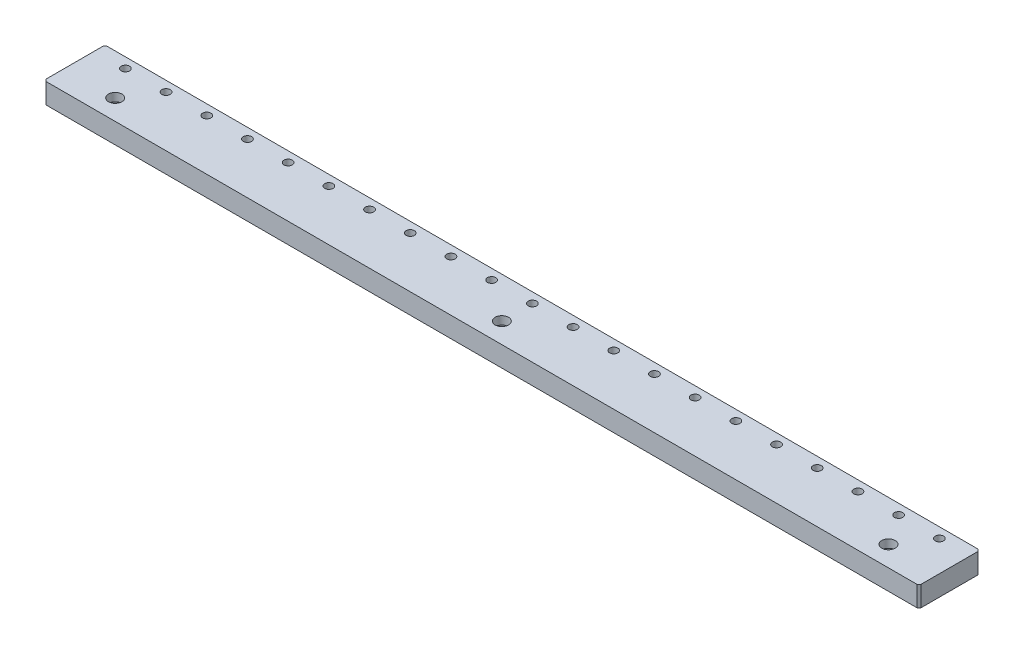
from build123d import *

# Parameters (mm, degrees)
SKETCH_1_W                  = 430
SKETCH_1_H                  = 30
EXTRUDE_1_DEPTH             = 5
CHAMFER_1_SIZE              = 1
HOLE_WIZARD_1_D             = 6.6
HOLE_WIZARD_1_CBORE_D       = 11
HOLE_WIZARD_1_CBORE_DEPTH   = 6
HOLE_WIZARD_4_1_4_1_1_D     = 4.1
HOLE_WIZARD_4_1_4_1_1_DEPTH = 10
HOLE_WIZARD_4_1_4_1_1_TIP   = 1.231764269


with BuildPart() as part:
    # 草图1 → 凸台-拉伸1 (new, symmetric)
    with BuildSketch(Plane(origin=(0, 0, 0), x_dir=(1, 0, 0), z_dir=(0, 1, 0))):
        Rectangle(SKETCH_1_W, SKETCH_1_H)
    extrude(amount=EXTRUDE_1_DEPTH, both=True)

    # 倒角1
    chamfer_1_edges = [part.edges().sort_by_distance(p)[0] for p in [
        (215, 0, 15),
        (-215, 0, 15),
        (-215, 0, -15),
        (215, 0, -15),
    ]]
    chamfer(chamfer_1_edges, length=CHAMFER_1_SIZE)

    # 打孔尺寸(%根据)内六角圆柱头螺钉的类型1 (through all)
    with Locations(Plane(origin=(0, -5, 0), x_dir=(-1, 0, 0), z_dir=(0, -1, 0))):
        with Locations((-190, -5), (0, -5), (190, -5)):
            CounterBoreHole(HOLE_WIZARD_1_D / 2, HOLE_WIZARD_1_CBORE_D / 2, HOLE_WIZARD_1_CBORE_DEPTH)

    # Ø4.1 (4.1) 直径孔1
    with Locations(Plane(origin=(0, -5, -18.75), x_dir=(-1, 0, 0), z_dir=(0, -1, 0))):
        with Locations((-200, -8.75), (-180, -8.75), (-160, -8.75), (-140, -8.75), (-120, -8.75), (-100, -8.75), (-80, -8.75), (-60, -8.75), (-40, -8.75), (-20, -8.75), (0, -8.75), (20, -8.75), (40, -8.75), (60, -8.75), (80, -8.75), (100, -8.75), (120, -8.75), (140, -8.75), (160, -8.75), (180, -8.75), (200, -8.75)):
            Hole(HOLE_WIZARD_4_1_4_1_1_D / 2, depth=HOLE_WIZARD_4_1_4_1_1_DEPTH)
            with Locations((0, 0, -(HOLE_WIZARD_4_1_4_1_1_DEPTH + HOLE_WIZARD_4_1_4_1_1_TIP / 2))):  # 118° drill point
                Cone(0, HOLE_WIZARD_4_1_4_1_1_D / 2, HOLE_WIZARD_4_1_4_1_1_TIP, mode=Mode.SUBTRACT)


solid = part.part
